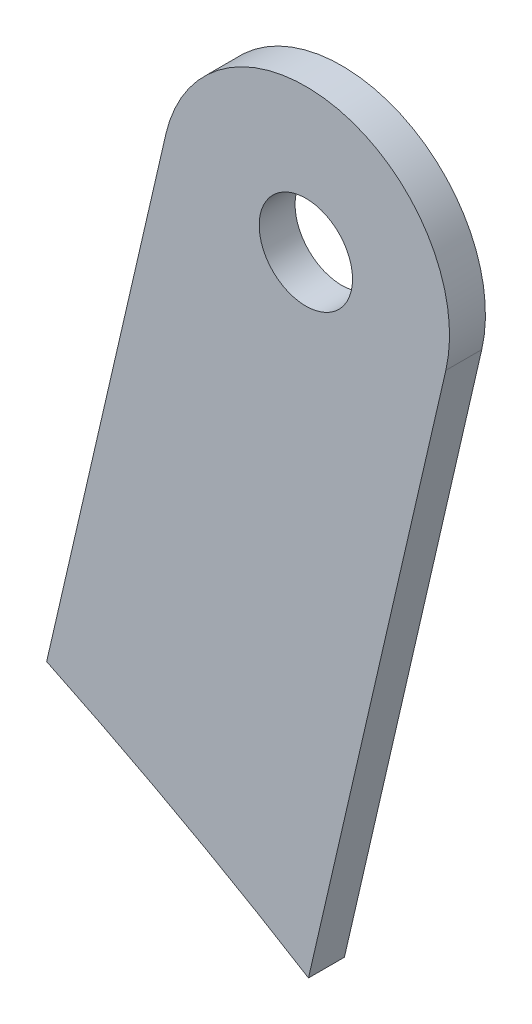
SolidWorks part; units mm, degrees
material "钢板5/Q235A "
ref_plane "Front Plane" through (0, 0, 0) normal (0, 0, 1) x (1, 0, 0)
ref_plane "Top Plane" through (0, 0, 0) normal (0, 1, 0) x (1, 0, 0)
ref_plane "Right Plane" through (0, 0, 0) normal (1, 0, 0) x (0, 0, -1)
sketch "Sketch1" plane through (0, 0, 0) normal (0, 0, 1) x (1, 0, 0)
  line L0 (167.313, 349.5177) -> (183.9126, 421.4184)
  line L1 (203.7666, 329.5989) -> (222.8874, 412.4204)
  line L2 (0, 0) -> (0, 499.5125) construction
  circle A0 centre (0, 0) radius 387.5 construction
  arc A1 (167.313, 349.5177) -> (203.7666, 329.5989) centre (0, 0) cw
  arc A2 (183.9126, 421.4184) -> (222.8874, 412.4204) centre (203.4, 416.9194) cw
  circle A3 centre (203.4, 416.9194) radius 6.5
  dimension "D1" = 775
  dimension "D2" = 20
  dimension "D4" = 13
  dimension "D3" = 85
  dimension "D5" = 203.4
  dimension "D6" = 13
extrude "Boss-Extrude1" add sketch "Sketch1" along normal mid plane 5
